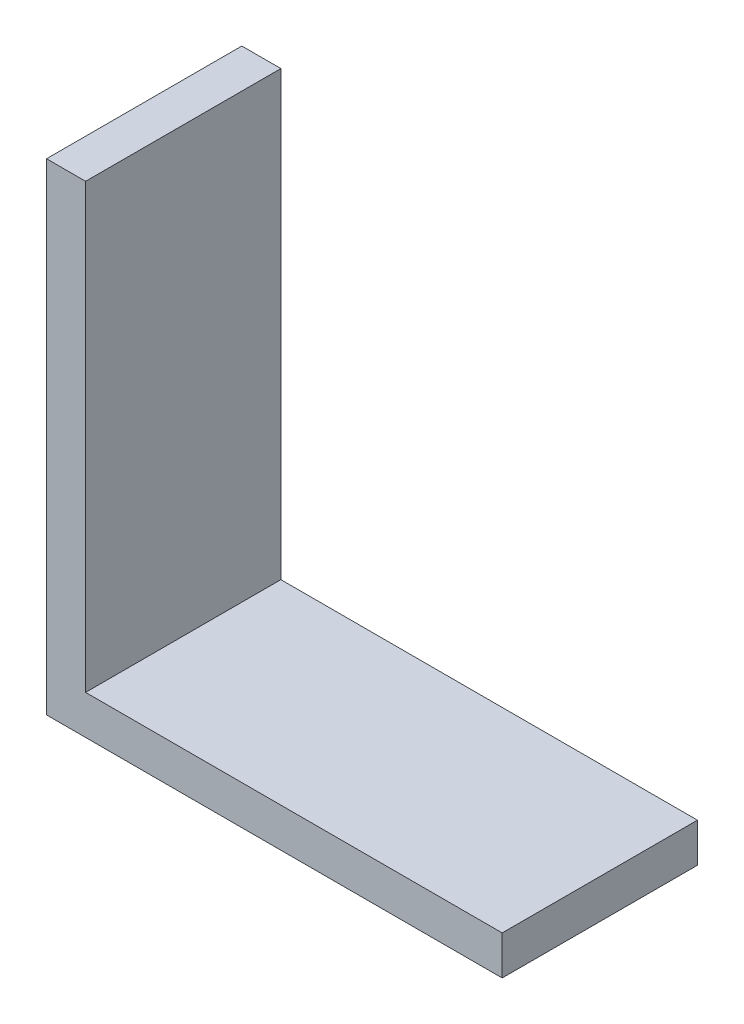
SolidWorks part; units mm, degrees
ref_plane "前视基准面" through (0, 0, 0) normal (0, 0, 1) x (1, 0, 0)
ref_plane "上视基准面" through (0, 0, 0) normal (0, 1, 0) x (1, 0, 0)
ref_plane "右视基准面" through (0, 0, 0) normal (1, 0, 0) x (0, 0, -1)
other "Configuration Table"
sketch "草图1" plane through (0, 0, 0) normal (0, 0, 1) x (1, 0, 0)
  line L0 (0, 0) -> (70, 0)
  line L1 (70, 0) -> (70, 6)
  line L2 (70, 6) -> (6, 6)
  line L3 (6, 6) -> (6, 74)
  line L4 (6, 74) -> (0, 74)
  line L5 (0, 74) -> (0, 0)
  point P0 (0, 0)
  dimension "D1" = 64
  dimension "D2" = 70
  dimension "D3" = 68
  dimension "D4" = 74
extrude "凸台-拉伸1" add sketch "草图1" against normal mid plane 30
